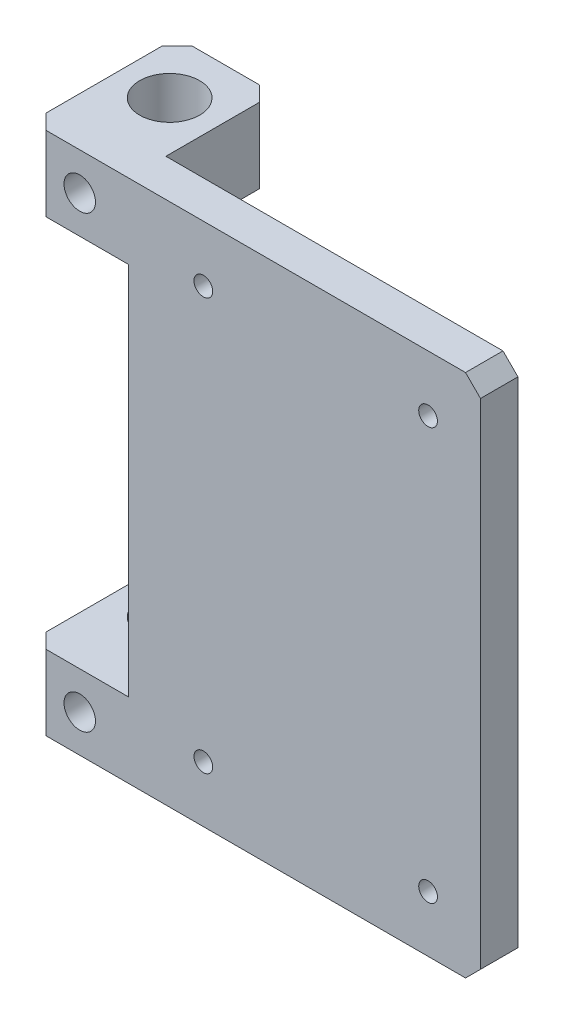
SolidWorks part; units mm, degrees
ref_plane "Front Plane" through (0, 0, 0) normal (0, 0, 1) x (1, 0, 0)
ref_plane "Top Plane" through (0, 0, 0) normal (0, 1, 0) x (1, 0, 0)
ref_plane "Right Plane" through (0, 0, 0) normal (1, 0, 0) x (0, 0, -1)
sketch "Sketch1" plane through (0, 0, 0) normal (0, 1, 0) x (1, 0, 0)
  line L1 (0, 0) -> (60, 0)
  line L2 (0, 0) -> (0, 25)
  line L3 (0, 25) -> (13, 25)
  line L4 (60, 0) -> (60, 5)
  line L7 (60, 5) -> (13, 5)
  line L8 (13, 25) -> (13, 5)
  dimension "D1" = 5
  dimension "D2" = 13
  dimension "D3" = 60
  dimension "D4" = 25
extrude "Boss-Extrude1" add sketch "Sketch1" along normal blind 70
sketch "Sketch2" plane through (0, 0, 0) normal (0, 0, 1) x (1, 0, 0)
  line L0 (0, 35) -> (50000, 35) construction
  line L1 (0, 70) -> (0, 0) construction
  line L2 (60, 70) -> (60, 0) construction
  circle A0 centre (53, 62.5) radius 0.75
  circle A1 centre (53, 7.5) radius 0.75
  point P4 (0, 35)
  dimension "D1" = 55
  dimension "D2" = 7
  dimension "D3" = 1.5
extrude "Cut-Extrude1" cut sketch "Sketch2" against normal blind 10
sketch "Sketch3" plane through (0, 0, 0) normal (-1, 0, 0) x (0, 0, 1)
  line L0 (-25, 35) -> (49975, 35) construction
  line L1 (-25, 70) -> (-25, 0) construction
  line L2 (0, 70) -> (0, 0) construction
  line L3 (-25, 60) -> (0, 60)
  line L4 (-25, 60) -> (-25, 10)
  line L5 (-25, 10) -> (0, 10)
  line L6 (0, 60) -> (0, 10)
  line L7 (-25, 60) -> (0, 10) construction
  line L8 (-25, 10) -> (0, 60) construction
  point P4 (-25, 35)
  point P5 (-12.5, 35)
  dimension "D1" = 50
extrude "Cut-Extrude2" cut sketch "Sketch3" against normal up to surface (13 mm away) up to face at (13, 35, -15)
sketch "Sketch4" plane through (0, 70, 0) normal (0, 1, 0) x (1, 0, 0)
  line L0 (6.5, 25) -> (6.5, -49975) construction
  line L1 (13, 25) -> (0, 25) construction
  line L2 (0, 12) -> (50000, 12) construction
  circle A0 centre (6.5, 12) radius 4
  point P4 (6.5, 25)
  dimension "D1" = 8
  dimension "D2" = 13
extrude "Cut-Extrude3" cut sketch "Sketch4" against normal through all
sketch "Sketch5" plane through (0, 0, 0) normal (0, 0, 1) x (1, 0, 0)
  line L1 (0, 60) -> (13, 60)
  line L2 (0, 60) -> (0, 10)
  line L3 (0, 10) -> (13, 10)
  line L4 (13, 60) -> (13, 10)
extrude "Boss-Extrude2" add sketch "Sketch5" against normal up to surface (5 mm away) up to face at (53.75, 7.5, -5)
sketch "Sketch9" plane through (0, 70, 0) normal (0, 1, 0) x (1, 0, 0)
  line L0 (13, 5) -> (13, 25) construction
  line L1 (0, 25) -> (13, 25)
  line L2 (0, 25) -> (0, 19.5)
  line L3 (0, 19.5) -> (13, 19.5)
  line L4 (13, 25) -> (13, 19.5)
  dimension "D1" = 5.5
extrude "Cut-Extrude6" cut sketch "Sketch9" against normal blind 71
pattern_linear "LPattern1" count 2 spacing 30 along (-1, 0, 0) of "Cut-Extrude1"
sketch "Sketch10" plane through (0, 0, -19.5) normal (0, 0, -1) x (-1, 0, 0)
  line L0 (0, 10) -> (0, 60) construction
  line L1 (-13, 10) -> (0, 10)
  line L2 (-13, 10) -> (-13, 60)
  line L3 (-13, 60) -> (0, 60)
  line L4 (0, 10) -> (0, 60)
extrude "Cut-Extrude7" cut sketch "Sketch10" against normal through all
chamfer "Chamfer1" distance 2 angle 45 6 edges at (0, 5, 0) (13, 5, -19.5) (0, 5, -19.5) (0, 65, 0) (13, 65, -19.5) (0, 65, -19.5)
chamfer "Chamfer2" distance 2 angle 45 2 edges at (60, 70, -2.5) (60, 0, -2.5)
hole_wizard "M3 Tapped Hole1" positions "3DSketch1" profile "Sketch11" tap size "M3" standard "Gb"
sketch3d "3DSketch1"
  line L0 (23, 7.5, -5) -> (23, 7.5, 0) construction
  line L1 (53, 7.5, -5) -> (53, 7.5, 0) construction
  line L2 (53, 62.5, -5) -> (53, 62.5, 0) construction
  line L3 (23, 62.5, -5) -> (23, 62.5, 0) construction
  point P0 (23, 7.5, -5)
  point P4 (53, 7.5, -5)
  point P8 (53, 62.5, -5)
  point P12 (23, 62.5, -5)
sketch "Sketch11" plane through (23, 7.5, -5) normal (1, 0, 0) x (0, 1, 0)
  line L0 (0, 0) -> (0, 8.2511)
  line L1 (0, 8.2511) -> (1.25, 7.5)
  line L2 (1.25, 7.5) -> (1.25, 0)
  line L5 (1.25, 0) -> (0, 0)
  line L10 (0, 8.2511) -> (-1.25, 7.5) construction
  line L11 (0, -6.35) -> (0, 107.95) construction
  dimension "螺纹孔钻头直径" = 2.5
  dimension "螺纹孔钻头深度" = 7.5
  dimension "导头角度" = 118
cosmetic thread "Hole Thread 1" parameters "D1"=5, "D2"=3
cosmetic thread "Hole Thread 2" parameters "D1"=5, "D2"=3
cosmetic thread "Hole Thread 3" parameters "D1"=5, "D2"=3
cosmetic thread "Hole Thread 4" parameters "D1"=5, "D2"=3
hole_wizard "M5 Tapped Hole1" positions "3DSketch2" profile "Sketch12" tap size "M5" standard "Gb"
sketch3d "3DSketch2"
  point P0 (6.5, 5, 0)
  dimension "D1" = 5
  dimension "D2" = 6.5
sketch "Sketch12" plane through (6.5, 5, 0) normal (1, 0, 0) x (0, -1, 0)
  line L0 (0, 0) -> (0, 13.6618)
  line L1 (0, 13.6618) -> (2.1, 12.4)
  line L2 (2.1, 12.4) -> (2.1, 0)
  line L5 (2.1, 0) -> (0, 0)
  line L10 (0, 13.6618) -> (-2.1, 12.4) construction
  line L11 (0, -6.35) -> (0, 107.95) construction
  dimension "螺纹孔钻头直径" = 4.2
  dimension "螺纹孔钻头深度" = 12.4
  dimension "导头角度" = 118
cosmetic thread "Hole Thread 5" parameters "D1"=8.5956, "D2"=5
hole_wizard "M5 Tapped Hole2" positions "3DSketch3" profile "Sketch13" tap size "M5" standard "Gb"
sketch3d "3DSketch3"
  line L0 (2, 70, 0) -> (58, 70, 0) construction
  point P0 (6.5, 65, 0)
  dimension "D1" = 5
  dimension "D2" = 6.5
sketch "Sketch13" plane through (6.5, 65, 0) normal (1, 0, 0) x (0, -1, 0)
  line L0 (0, 0) -> (0, 13.6618)
  line L1 (0, 13.6618) -> (2.1, 12.4)
  line L2 (2.1, 12.4) -> (2.1, 0)
  line L5 (2.1, 0) -> (0, 0)
  line L10 (0, 13.6618) -> (-2.1, 12.4) construction
  line L11 (0, -6.35) -> (0, 107.95) construction
  dimension "螺纹孔钻头直径" = 4.2
  dimension "螺纹孔钻头深度" = 12.4
  dimension "导头角度" = 118
cosmetic thread "Hole Thread 6" parameters "D1"=8.5956, "D2"=5
chamfer "Chamfer3" distance 0.8 angle 45 4 edges at (21.75, 62.5, -5) (51.75, 62.5, -5) (21.75, 7.5, -5) (51.75, 7.5, -5)
